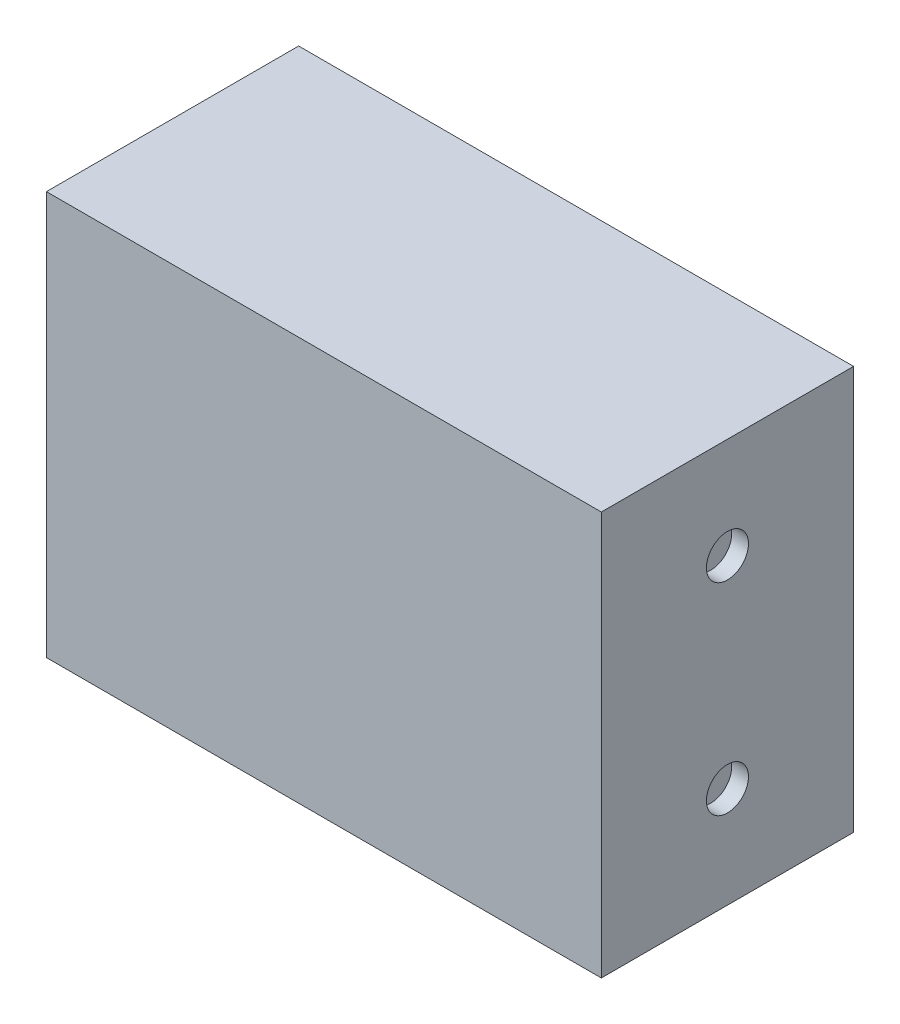
from build123d import *

# Parameters (mm, degrees)
SKETCH_1_W          = 330
SKETCH_1_H          = 240
EXTRUDE_1_DEPTH     = 150
SKETCH_2_R          = 12.5
CUT_EXTRUDE_1_DEPTH = 10
SKETCH_3_R          = 2.75
CUT_EXTRUDE_2_DEPTH = 10


with BuildPart() as part:
    # 草图1 → 凸台-拉伸1 (new body)
    with BuildSketch(Plane.XY):
        Rectangle(SKETCH_1_W, SKETCH_1_H)
    extrude(amount=EXTRUDE_1_DEPTH)

    # 草图2 → 切除-拉伸1 (cut)
    with BuildSketch(Plane(origin=(165, 0, 0), x_dir=(0, 0, -1), z_dir=(1, 0, 0))):
        with Locations(Location((-75, 60, 0), (0, 0, 90))):
            Circle(SKETCH_2_R)
        with Locations(Location((-75, -60, 0), (0, 0, 90))):
            Circle(SKETCH_2_R)
    extrude(amount=-CUT_EXTRUDE_1_DEPTH, mode=Mode.SUBTRACT)

    # 草图3 → 切除-拉伸2 (cut)
    with BuildSketch(Plane.ZY.offset(165)):
        with Locations(Location((40, 80, 0), (0, 0, 270))):
            Circle(SKETCH_3_R)
        with Locations(Location((110, 80, 0), (0, 0, 270))):
            Circle(SKETCH_3_R)
        with Locations(Location((110, -80, 0), (0, 0, 270))):
            Circle(SKETCH_3_R)
        with Locations(Location((40, -80, 0), (0, 0, 270))):
            Circle(SKETCH_3_R)
    extrude(amount=-CUT_EXTRUDE_2_DEPTH, mode=Mode.SUBTRACT)


solid = part.part
